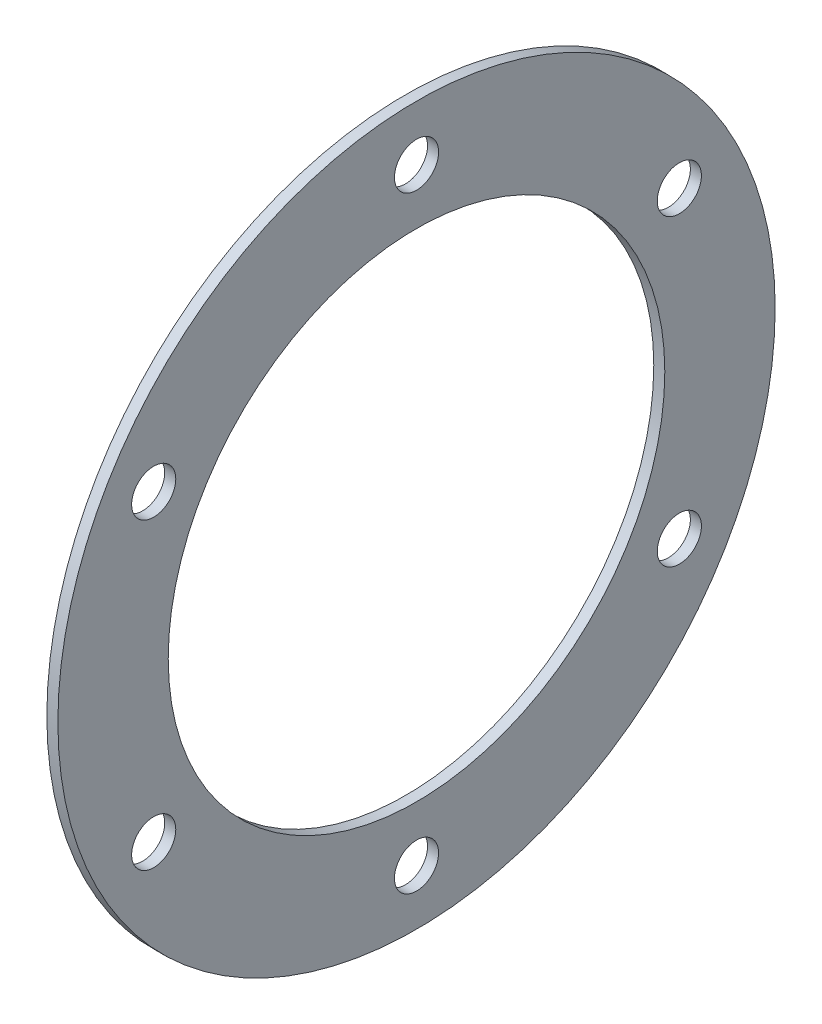
from build123d import *

# Parameters (mm, degrees)
SKETCH1_W          = 2
SKETCH1_H          = 20
SKETCH2_R          = 4
CUT_EXTRUDE1_DEPTH = 10
SCALE_1_SCALE      = 1.875


with BuildPart() as part:
    # Sketch1 → Revolve1 (revolve)
    with BuildSketch(Plane.XY, mode=Mode.PRIVATE) as revolve1_sk:
        with Locations((1, 55)):
            Rectangle(SKETCH1_W, SKETCH1_H)
    revolve(revolve1_sk.sketch.rotate(Axis((0, 0, 0), (1, 0, 0)), 90), axis=Axis((0, 0, 0), (1, 0, 0)))

    # Sketch2 → Cut-Extrude1 (cut)
    with BuildSketch(Plane(origin=(2, 0, 0), x_dir=(0, 0, -1), z_dir=(1, 0, 0))):
        with Locations((0, 55)):
            Circle(SKETCH2_R)
        with Locations((47.631397208, 27.5)):
            Circle(SKETCH2_R)
        with Locations((-47.631397208, 27.5)):
            Circle(SKETCH2_R)
        with Locations((47.631397208, -27.5)):
            Circle(SKETCH2_R)
        with Locations((-47.631397208, -27.5)):
            Circle(SKETCH2_R)
        with Locations((0, -55)):
            Circle(SKETCH2_R)
    extrude(amount=-CUT_EXTRUDE1_DEPTH, mode=Mode.SUBTRACT)


with BuildPart() as part_1:
    # Scale 1: scaled about (1, 0, 0)
    add(part.part.scale(SCALE_1_SCALE).moved(Location((-0.875, 0, 0))))


solid = part_1.part
